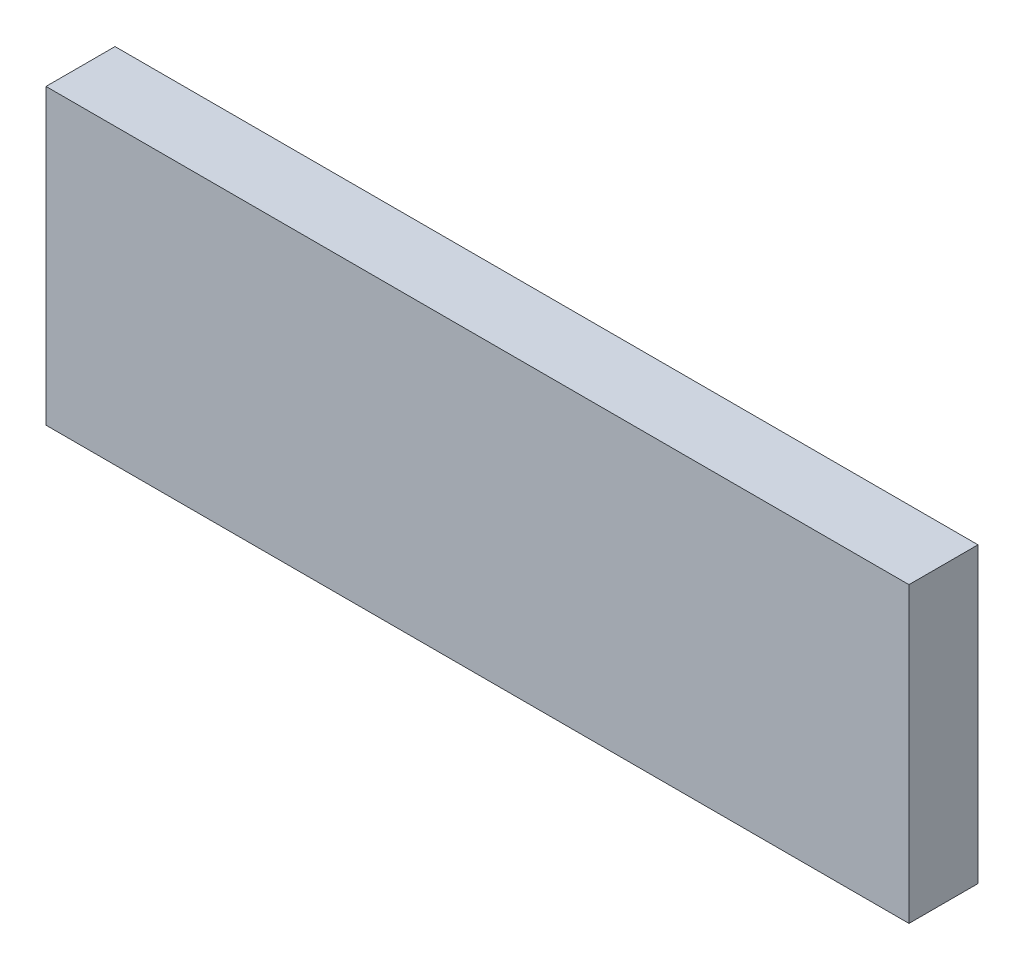
SolidWorks part; units mm, degrees
material "Q235"
ref_plane "Front Plane" through (0, 0, 0) normal (0, 0, 1) x (1, 0, 0)
ref_plane "Top Plane" through (0, 0, 0) normal (0, 1, 0) x (1, 0, 0)
ref_plane "Right Plane" through (0, 0, 0) normal (1, 0, 0) x (0, 0, -1)
sketch "Sketch1" plane through (0, 0, 0) normal (0, 0, 1) x (1, 0, 0)
  line L1 (0, 0) -> (200, 0)
  line L2 (0, 0) -> (0, 68)
  line L3 (0, 68) -> (200, 68)
  line L4 (200, 0) -> (200, 68)
  dimension "D1" = 200
  dimension "D2" = 68
extrude "Boss-Extrude1" add sketch "Sketch1" along normal blind 16
